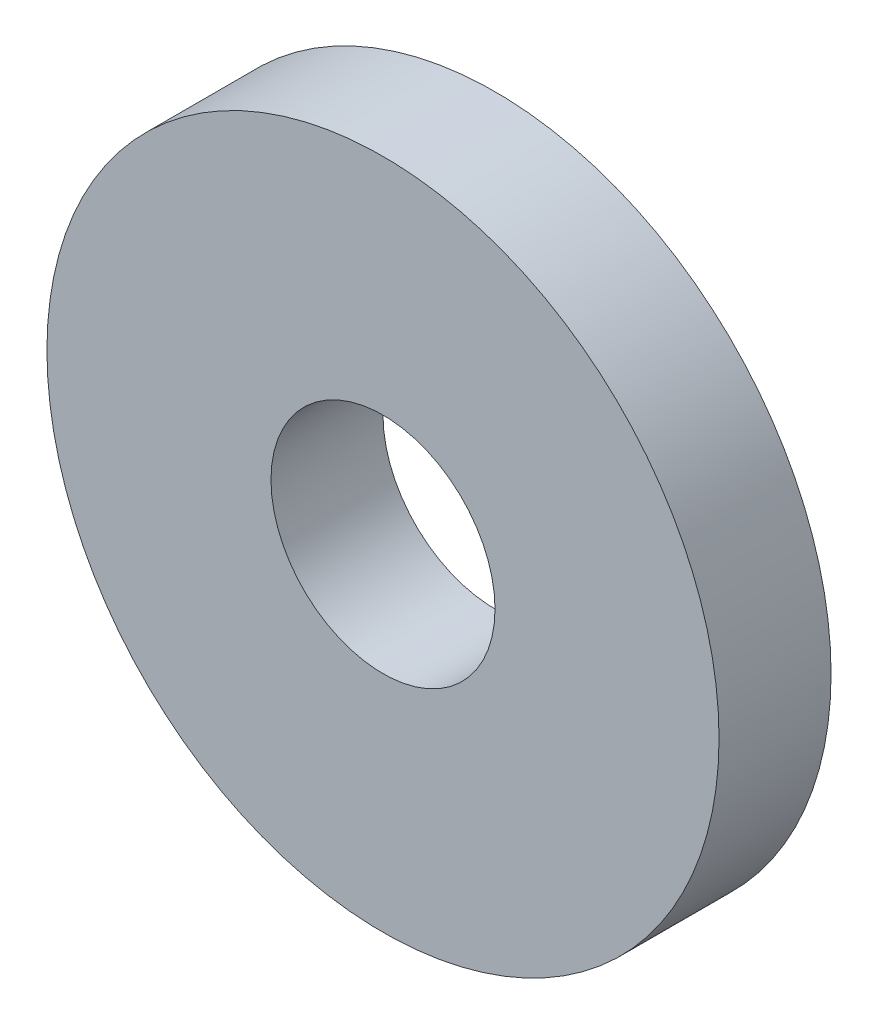
SolidWorks part; units mm, degrees
ref_plane "前视基准面" through (0, 0, 0) normal (0, 0, 1) x (1, 0, 0)
ref_plane "上视基准面" through (0, 0, 0) normal (0, 1, 0) x (1, 0, 0)
ref_plane "右视基准面" through (0, 0, 0) normal (1, 0, 0) x (0, 0, -1)
other "Configuration Table"
sketch "草图1" plane through (0, 0, 0) normal (0, 0, 1) x (1, 0, 0)
  circle A0 centre (0, 0) radius 6
  circle A1 centre (0, 0) radius 2
extrude "凸台-拉伸1" add sketch "草图1" along normal blind 2
